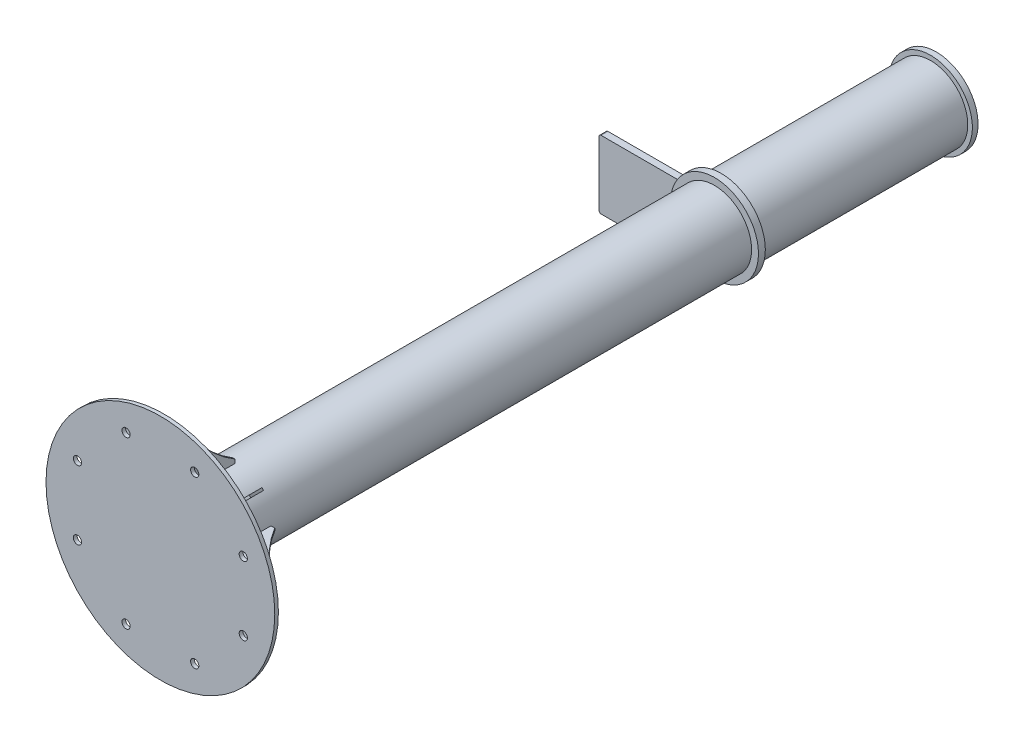
from build123d import *

# Parameters (mm, degrees)
SKETCH1_R           = 162.5
SKETCH1_R_2         = 142.5
BOSS_EXTRUDE1_DEPTH = 3363.5
BOSS_EXTRUDE2_START = -2436
SKETCH2_R           = 192.5
SKETCH2_R_2         = 162.5
BOSS_EXTRUDE2_DEPTH = 30
SKETCH3_R           = 500
BOSS_EXTRUDE3_DEPTH = 16
BOSS_EXTRUDE4_DEPTH = 5
CIRPATTERN1_COUNT   = 8
SKETCH5_R           = 18
CUT_EXTRUDE1_DEPTH  = 3438.023749
SKETCH6_R           = 182.5
BOSS_EXTRUDE5_DEPTH = 12.5
BOSS_EXTRUDE6_START = -895
BOSS_EXTRUDE6_DEPTH = 30


with BuildPart() as part:
    # Sketch1 → Boss-Extrude1 (new body)
    with BuildSketch(Plane.XY):
        Circle(SKETCH1_R)
        Circle(SKETCH1_R_2, mode=Mode.SUBTRACT)
    extrude(amount=BOSS_EXTRUDE1_DEPTH)

    # Sketch2 → Boss-Extrude2 (add)
    with BuildSketch(Plane.XY.offset(3363.5).offset(BOSS_EXTRUDE2_START)):
        Circle(SKETCH2_R)
        Circle(SKETCH2_R_2, mode=Mode.SUBTRACT)
    extrude(amount=BOSS_EXTRUDE2_DEPTH)

    # Sketch3 → Boss-Extrude3 (add)
    with BuildSketch(Plane.XY.offset(3363.5)):
        Circle(SKETCH3_R)
    extrude(amount=BOSS_EXTRUDE3_DEPTH)

    # Sketch4 → Boss-Extrude4 (add, symmetric)
    with BuildSketch(Plane(origin=(0, 0, 0), x_dir=(0, 0, -1), z_dir=(1, 0, 0))):
        with BuildLine():
            Line((-3058.5, 150.103779), (-3058.5, 179.159054))
            ThreePointArc((-3058.5, 179.159054), (-3169.176272, 266.043477), (-3255.057488, 377.5))
            Line((-3255.057488, 377.5), (-3363.5, 377.5))
            Line((-3363.5, 377.5), (-3363.5, 150.103779))
            Line((-3363.5, 150.103779), (-3058.5, 150.103779))
        make_face()
    boss_extrude4 = extrude(amount=BOSS_EXTRUDE4_DEPTH, both=True)

    # CirPattern1: Boss-Extrude4 ×8 about axis
    cirpattern1_axis = Axis((0, 0, 0), (0, 0, 1))
    for i in range(1, CIRPATTERN1_COUNT):
        add(boss_extrude4.rotate(cirpattern1_axis, i * 360 / CIRPATTERN1_COUNT))

    # Sketch5 → Cut-Extrude1 (cut, through all)
    with BuildSketch(Plane(origin=(0, 0, 3363.5), x_dir=(-1, 0, 0), z_dir=(0, 0, -1))):
        with Locations((150.144602, 362.481135)):
            Circle(SKETCH5_R)
        with Locations((362.481135, 150.144602)):
            Circle(SKETCH5_R)
        with Locations((362.481135, -150.144602)):
            Circle(SKETCH5_R)
        with Locations((150.144602, -362.481135)):
            Circle(SKETCH5_R)
        with Locations((-150.144602, -362.481135)):
            Circle(SKETCH5_R)
        with Locations((-362.481135, -150.144602)):
            Circle(SKETCH5_R)
        with Locations((-362.481135, 150.144602)):
            Circle(SKETCH5_R)
        with Locations((-150.144602, 362.481135)):
            Circle(SKETCH5_R)
    extrude(amount=-CUT_EXTRUDE1_DEPTH, mode=Mode.SUBTRACT)

    # Sketch6 → Boss-Extrude5 (add, symmetric)
    with BuildSketch(Plane(origin=(0, 0, 0), x_dir=(-1, 0, 0), z_dir=(0, 0, -1))):
        Circle(SKETCH6_R)
    extrude(amount=BOSS_EXTRUDE5_DEPTH, both=True)

    # Sketch7 → Boss-Extrude6 (add)
    with BuildSketch(Plane(origin=(0, 0, -12.5), x_dir=(-1, 0, 0), z_dir=(0, 0, -1)).offset(BOSS_EXTRUDE6_START)):
        with BuildLine():
            Line((129.712181, 59), (540, 59))
            ThreePointArc((540, 59), (547.071068, 56.071068), (550, 49))
            Line((550, 49), (550, 0))
            Line((550, 0), (550, -229))
            ThreePointArc((550, -229), (547.071068, -236.071068), (540, -239))
            Line((540, -239), (267.25882, -239))
            ThreePointArc((267.25882, -239), (260.187752, -236.071068), (257.25882, -229))
            Line((257.25882, -229), (257.25882, -99))
            ThreePointArc((257.25882, -99), (245.543091, -70.715729), (217.25882, -59))
            Line((217.25882, -59), (129.712181, -59))
            ThreePointArc((129.712181, -59), (142.5, 0), (129.712181, 59))
        make_face()
    extrude(amount=-BOSS_EXTRUDE6_DEPTH)


solid = part.part
